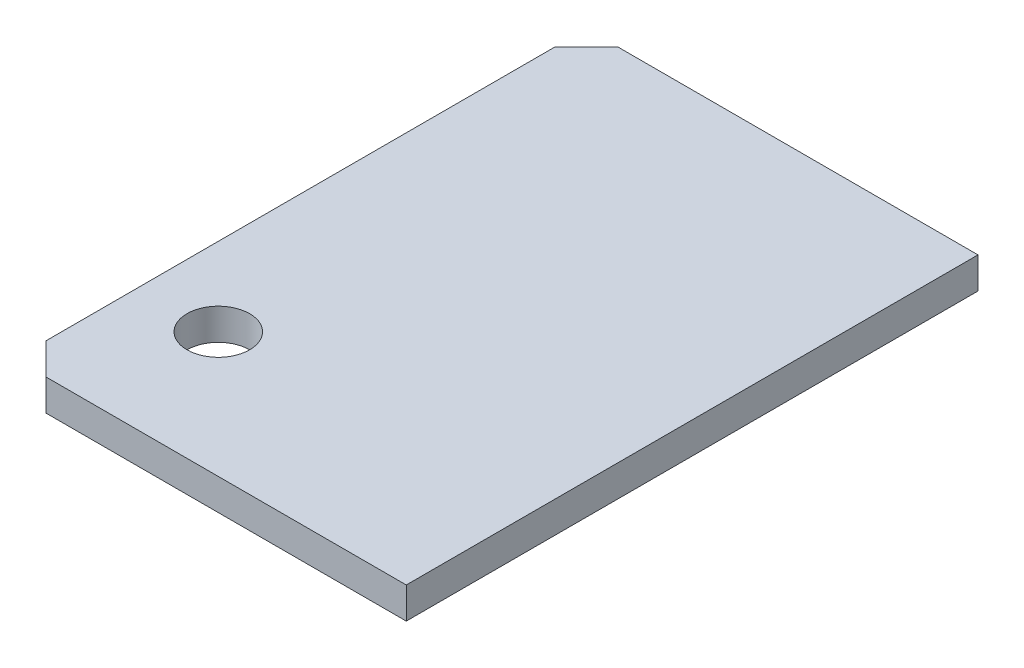
SolidWorks part; units mm, degrees
ref_plane "Front Plane" through (0, 0, 0) normal (0, 0, 1) x (1, 0, 0)
ref_plane "Top Plane" through (0, 0, 0) normal (0, 1, 0) x (1, 0, 0)
ref_plane "Right Plane" through (0, 0, 0) normal (1, 0, 0) x (0, 0, -1)
sketch "Sketch1" plane through (0, 0, 0) normal (0, 0, 1) x (1, 0, 0)
  line L1 (0, 0) -> (-250, 0)
  line L2 (0, 0) -> (0, 20)
  line L3 (0, 20) -> (-250, 20)
  line L4 (-250, 0) -> (-250, 20)
  dimension "D1" = 250
  dimension "D2" = 20
extrude "Boss-Extrude1" add sketch "Sketch1" along normal blind 365
chamfer "Chamfer1" distance 20 angle 45 1 edges at (-250, 10, 365)
sketch "Sketch2" plane through (0, 20, 0) normal (0, 1, 0) x (1, 0, 0)
  line L0 (0, -365) -> (-230, -365) construction
  line L1 (-250, -345) -> (-250, 0) construction
  circle A0 centre (-200, -285) radius 20
  dimension "D1" = 40
  dimension "D2" = 80
  dimension "D3" = 50
extrude "Cut-Extrude1" cut sketch "Sketch2" against normal through all both and the other way through all
chamfer "Chamfer2" distance 20 angle 45 1 edges at (-250, 10, 0)
